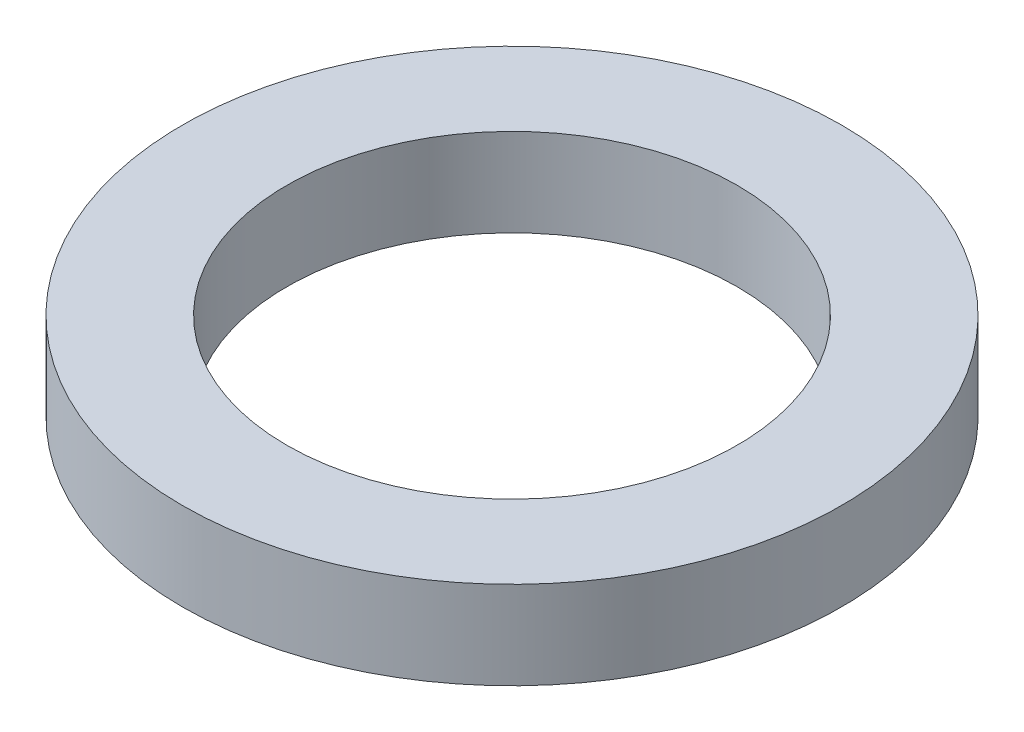
SolidWorks part; units mm, degrees
ref_plane "Front Plane" through (0, 0, 0) normal (0, 0, 1) x (1, 0, 0)
ref_plane "Top Plane" through (0, 0, 0) normal (0, 1, 0) x (1, 0, 0)
ref_plane "Right Plane" through (0, 0, 0) normal (1, 0, 0) x (0, 0, -1)
sketch "Sketch1" plane through (0, 0, 0) normal (0, 1, 0) x (1, 0, 0)
  circle A0 centre (0, 0) radius 6
  circle A1 centre (0, 0) radius 4.1
  dimension "D1" = 8.2
  dimension "D2" = 12
extrude "Boss-Extrude1" add sketch "Sketch1" along normal blind 1.6
